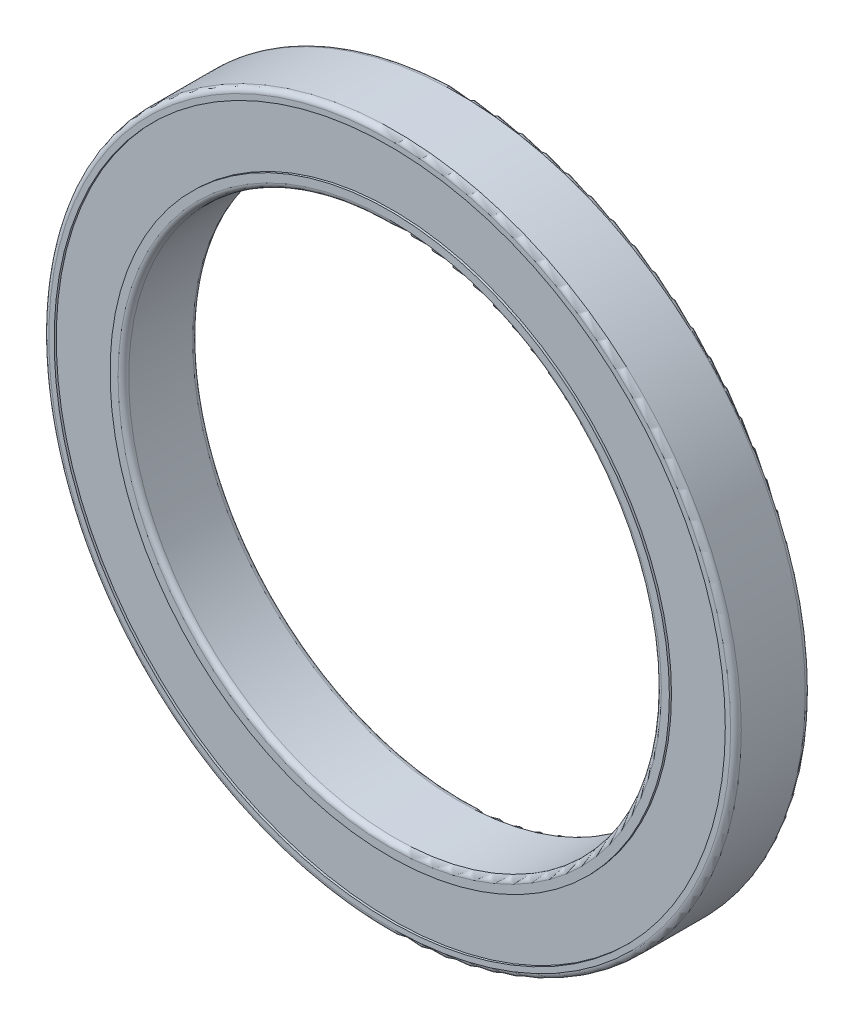
from build123d import *

# Parameters (mm, degrees)
SKETCH1_R           = 32.5
SKETCH1_R_2         = 25
BOSS_EXTRUDE1_DEPTH = 3.5
SKETCH2_R           = 31.5
SKETCH2_R_2         = 26.25
CUT_EXTRUDE1_DEPTH  = 0.2
FILLET1_R           = 0.5


with BuildPart() as part:
    # Sketch1 → Boss-Extrude1 (new, symmetric)
    with BuildSketch(Plane.XY):
        Circle(SKETCH1_R)
        Circle(SKETCH1_R_2, mode=Mode.SUBTRACT)
    extrude(amount=BOSS_EXTRUDE1_DEPTH, both=True)

    # Sketch2 → Cut-Extrude1 (cut)
    with BuildSketch(Plane.XY.offset(3.5)):
        Circle(SKETCH2_R)
        Circle(SKETCH2_R_2, mode=Mode.SUBTRACT)
    cut_extrude1 = extrude(amount=-CUT_EXTRUDE1_DEPTH, mode=Mode.SUBTRACT)

    # Mirror1: Cut-Extrude1 across plane
    add(cut_extrude1.mirror(Plane.XY), mode=Mode.SUBTRACT)

    # Fillet1
    fillet1_edges = [part.edges().sort_by_distance(p)[0] for p in [
        (-32.5, 0, -3.5),
        (-32.5, 0, 3.5),
        (-25, 0, -3.5),
        (-25, 0, 3.5),
    ]]
    fillet(fillet1_edges, radius=FILLET1_R)


solid = part.part
